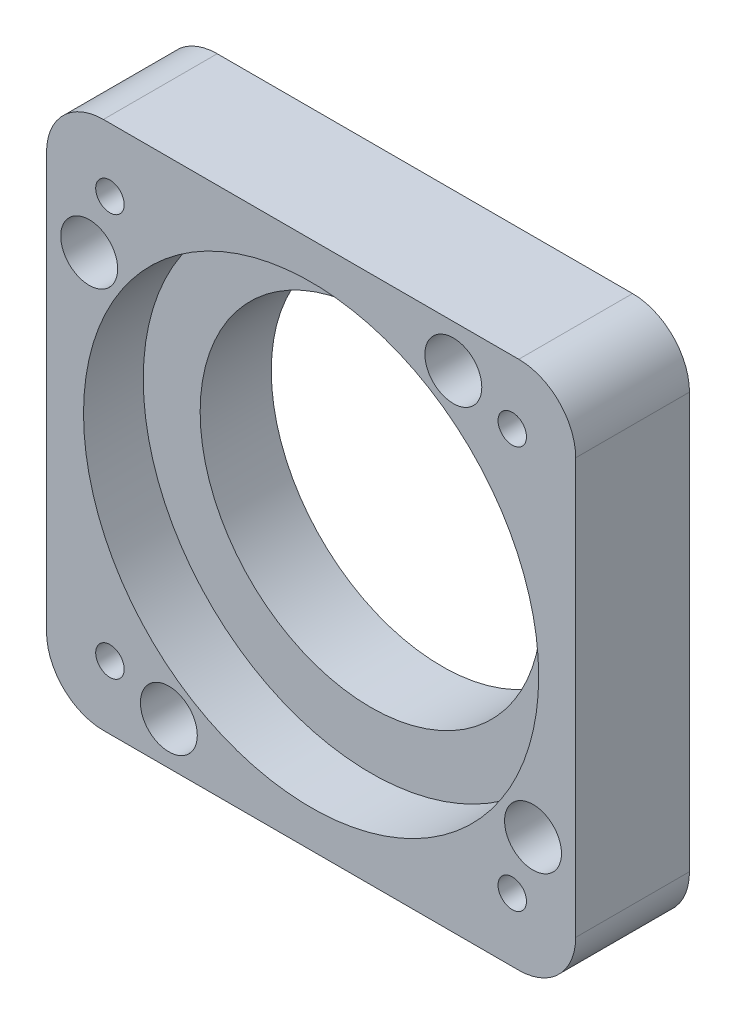
SolidWorks part; units mm, degrees
ref_plane "Front Plane" through (0, 0, 0) normal (0, 0, 1) x (1, 0, 0)
ref_plane "Top Plane" through (0, 0, 0) normal (0, 1, 0) x (1, 0, 0)
ref_plane "Right Plane" through (0, 0, 0) normal (1, 0, 0) x (0, 0, -1)
sketch "Sketch1" plane through (0, 0, 0) normal (0, 0, 1) x (1, 0, 0)
  line L1 (-46.5, -46.5) -> (46.5, -46.5)
  line L2 (-46.5, -46.5) -> (-46.5, 46.5)
  line L3 (-46.5, 46.5) -> (46.5, 46.5)
  line L4 (46.5, -46.5) -> (46.5, 46.5)
  line L5 (-46.5, -46.5) -> (46.5, 46.5) construction
  line L6 (-46.5, 46.5) -> (46.5, -46.5) construction
  circle A0 centre (0, 0) radius 30
  point P0 (0, 0)
  dimension "D3" = 60
  dimension "D1" = 93
  dimension "D2" = 93
extrude "Boss-Extrude1" add sketch "Sketch1" along normal blind 20
fillet "Fillet1" radius 10 4 edges at (-46.5, -46.5, 10) (46.5, -46.5, 10) (46.5, 46.5, 10) (-46.5, 46.5, 10)
sketch "Sketch6" plane through (0, 0, 0) normal (0, 0, -1) x (-1, 0, 0)
  circle A0 centre (0, 0) radius 30 construction
  circle A1 centre (0, 0) radius 30
  circle A2 centre (0, 0) radius 41
  dimension "D1" = 82
extrude "Boss-Extrude2" add sketch "Sketch6" along normal blind 3
sketch "Sketch7" plane through (0, 0, 20) normal (0, 0, 1) x (1, 0, 0)
  circle A0 centre (0, 0) radius 40
  dimension "D1" = 80
extrude "Cut-Extrude1" cut sketch "Sketch7" against normal blind 10.5
hole_wizard "M6 Tapped Hole1" positions "Sketch8" profile "Sketch9" tap size "M6" standard "GB" end condition through all
sketch "Sketch8" plane through (0, 0, 20) normal (0, 0, 1) x (1, 0, 0)
  line L0 (0, 0) -> (0, 50)
  line L1 (0, 0) -> (-50, 0)
  line L2 (-35.3553, 35.3553) -> (0, 0)
  circle A0 centre (0, 0) radius 50
  point P0 (-35.3553, 35.3553)
  point P24 (35.3553, 35.3553)
  point P25 (35.3553, -35.3553)
  point P26 (-35.3553, -35.3553)
  dimension "D1" = 100
  dimension "D2" = 45
cosmetic thread "Cosmetic Thread 1" parameters "D2"=6
cosmetic thread "Cosmetic Thread 2" parameters "D2"=6
cosmetic thread "Cosmetic Thread 3" parameters "D2"=6
cosmetic thread "Cosmetic Thread 4" parameters "D2"=6
sketch "Sketch9" plane through (-35.3553, 35.3553, 20) normal (1, 0, 0) x (0, -1, 0)
  line L0 (0, 0) -> (0, 23)
  line L1 (0, 23) -> (2.5, 23)
  line L2 (2.5, 23) -> (2.5, 0)
  line L5 (2.5, 0) -> (0, 0)
  line L11 (0, -6.35) -> (0, 107.95) construction
  dimension "通孔螺纹孔钻头直径" = 5
  dimension "通孔螺纹孔钻头深度" = 23
hole_wizard "CBORE for M5 Hex Head Bolt1" positions "Sketch5" profile "Sketch4" counterbore size "M5" standard "GB"
sketch "Sketch5" plane through (0, 0, 9.5) normal (0, 0, 1) x (1, 0, 0)
  line L0 (0, 0) -> (0, 32.5)
  circle A0 centre (0, 0) radius 32.5
  point P0 (0, 32.5)
  dimension "D1" = 65
sketch "Sketch4" plane through (0, 32.5, 9.5) normal (1, 0, 0) x (0, -1, 0)
  line L0 (0, 0) -> (0, 12.5)
  line L1 (0, 12.5) -> (2.75, 12.5)
  line L3 (2.75, 12.5) -> (2.75, 6)
  line L4 (2.75, 6) -> (4.5, 6)
  line L5 (4.5, 6) -> (4.5, 0)
  line L7 (4.5, 0) -> (0, 0)
  line L11 (0, -6.35) -> (0, 107.95) construction
  dimension "通孔孔直径" = 5.5
  dimension "通孔孔深度" = 12.5
  dimension "柱形沉头孔直径" = 9
  dimension "柱形沉头孔深度" = 6
pattern_circular "CirPattern1" [suppressed] count 4 every 90
hole_wizard "Hole Spec (per socket head cap screw type) 1" positions "Sketch10" profile "Sketch11" counterbore size "M5" standard "GB" end condition through all
sketch "Sketch10" plane through (0, 0, 20) normal (0, 0, 1) x (1, 0, 0)
  point P0 (-25, -39)
  dimension "D1" = 25
  dimension "D2" = 39
sketch "Sketch11" plane through (-25, -39, 20) normal (1, 0, 0) x (0, -1, 0)
  line L0 (0, 0) -> (0, 23)
  line L1 (0, 23) -> (2.75, 23)
  line L3 (2.75, 23) -> (2.75, 9.7)
  line L4 (2.75, 9.7) -> (5, 9.7)
  line L5 (5, 9.7) -> (5, 0)
  line L7 (5, 0) -> (0, 0)
  line L11 (0, -6.35) -> (0, 107.95) construction
  dimension "通孔孔直径" = 5.5
  dimension "通孔孔深度" = 23
  dimension "柱形沉头孔直径" = 10
  dimension "柱形沉头孔深度" = 9.7
pattern_circular "CirPattern2" count 4 every 90 about axis through (0, 0, 0) along (0, 0, 1) of "Hole Spec (per socket head cap screw type) 1"
